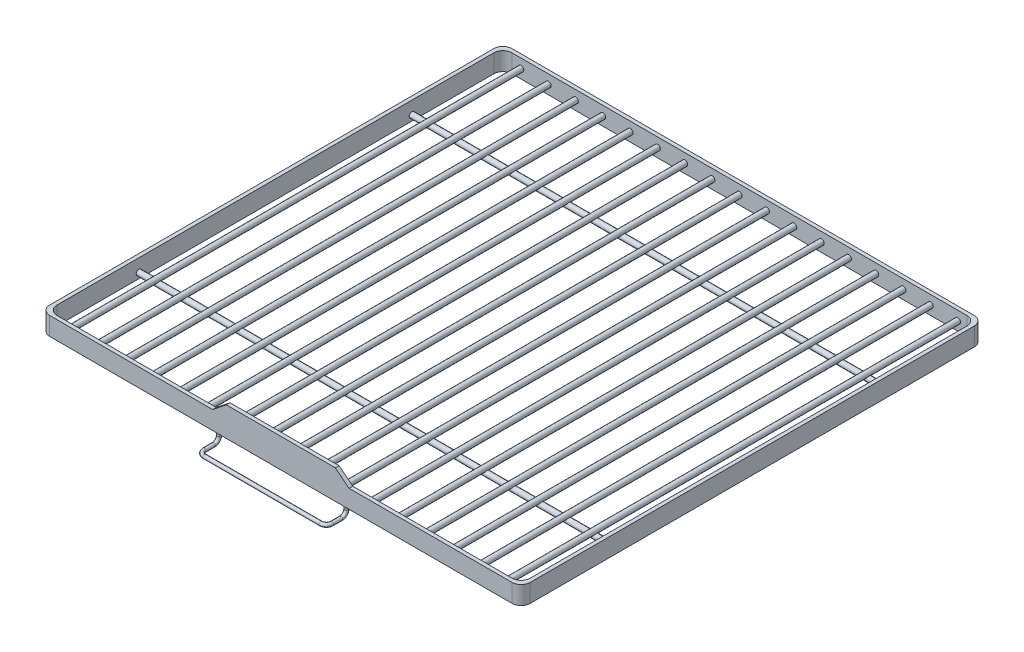
from build123d import *
from build123d.topology import SkipClean

# Parameters (mm, degrees)
SKETCH1_W           = 528
SKETCH1_H           = 508
SKETCH1_W_2         = 520
SKETCH1_H_2         = 500
BOSS_EXTRUDE1_DEPTH = 20
BOSS_EXTRUDE2_DEPTH = 4
FILLET1_R           = 10
SKETCH3_R           = 3
BOSS_EXTRUDE3_DEPTH = 520
BOSS_EXTRUDE4_REACH = 571.856
SKETCH4_R           = 3
LPATTERN1_COUNT     = 9
LPATTERN1_PITCH     = 30
LPATTERN2_COUNT     = 9
LPATTERN2_PITCH     = 30
SWEEP1_PROFILE_R    = 2
SWEEP2_PROFILE_R    = 2


with BuildPart() as part:
    # Sketch1 → Boss-Extrude1 (new body)
    with BuildSketch(Plane(origin=(0, 0, 0), x_dir=(1, 0, 0), z_dir=(0, 1, 0))):
        Rectangle(SKETCH1_W, SKETCH1_H)
        Rectangle(SKETCH1_W_2, SKETCH1_H_2, mode=Mode.SUBTRACT)
    extrude(amount=BOSS_EXTRUDE1_DEPTH)

    # Sketch2 → Boss-Extrude2 (add)
    with BuildSketch(Plane.XY.offset(254)):
        Polygon((60, 32), (-60, 32), (-75, 20), (75, 20), align=None)
    extrude(amount=-BOSS_EXTRUDE2_DEPTH)

    # Fillet1
    fillet1_edges = [part.edges().sort_by_distance(p)[0] for p in [
        (260, 10, 250),
        (260, 10, -250),
        (-260, 10, -250),
        (-260, 10, 250),
        (264, 10, -254),
        (264, 10, 254),
        (-264, 10, 254),
        (-264, 10, -254),
    ]]
    fillet(fillet1_edges, radius=FILLET1_R)

    # Sketch3 → Boss-Extrude3 (add)
    with BuildSketch(Plane(origin=(-260, 0, 0), x_dir=(0, 0, -1), z_dir=(1, 0, 0))):
        with Locations(Location((-150, 6, 0), (0, 0, 180))):
            Circle(SKETCH3_R)
        with Locations(Location((150, 6, 0), (0, 0, 180))):
            Circle(SKETCH3_R)
    extrude(amount=BOSS_EXTRUDE3_DEPTH)

    # Boss-Extrude4: up to this face of the body (flat: up to its plane)
    boss_extrude4_end = Plane(part.part.faces().sort_by_distance((0, 12.199655766, 250))[0])
    # Sketch4 → Boss-Extrude4 (add, up to the picked face)
    with BuildSketch(Plane.XY.offset(-250), mode=Mode.PRIVATE) as boss_extrude4_sk1:
        with Locations(Location((0, 10, 0), (0, 0, 180))):
            Circle(SKETCH4_R)
    boss_extrude4_tool1 = split(extrude(boss_extrude4_sk1.sketch, amount=BOSS_EXTRUDE4_REACH, mode=Mode.PRIVATE), bisect_by=boss_extrude4_end, keep=Keep.BOTH, mode=Mode.PRIVATE)
    boss_extrude4 = boss_extrude4_tool1.solids().sort_by(Axis((0, 10, -250), (0, 0, 1)))[0]
    add(boss_extrude4)

    # LPattern1: Boss-Extrude4 ×9
    with Locations(*[(i * LPATTERN1_PITCH, 0, 0) for i in range(1, LPATTERN1_COUNT)]):
        add(boss_extrude4)

    # LPattern2: Boss-Extrude4 ×9
    with Locations(*[(-i * LPATTERN2_PITCH, 0, 0) for i in range(1, LPATTERN2_COUNT)]):
        add(boss_extrude4)

    # Sweep1: sweep along a path in Sketch5
    with BuildLine(Plane(origin=(70, 0, 0), x_dir=(0, 0, -1), z_dir=(1, 0, 0))) as sweep1_path:
        Line((-252, 0), (-252, -3))
        ThreePointArc((-252, -3), (-253.757359313, -7.242640687), (-258, -9))
        Line((-258, -9), (-264, -9))
    # Sweep1 profile (on start of the path) → Sweep1 (sweep)
    with BuildSketch(Plane(origin=(70, 0, 252), x_dir=(0, 0, -1), z_dir=(0, -1, 0))):
        Circle(SWEEP1_PROFILE_R)
    sweep1 = sweep(path=sweep1_path.line)

    # Mirror1: Sweep1 across plane
    add(sweep1.mirror(Plane(origin=(0, 0, 0), x_dir=(0, 0, 1), z_dir=(1, 0, 0))))

    # Sweep2: sweep along a path in Sketch43
    with SkipClean():  # the faces are left unmerged after this step: merging them gives an invalid solid
        with BuildLine(Plane(origin=(0, -9, 0), x_dir=(1, 0, 0), z_dir=(0, 1, 0))) as sweep2_path:
            Line((-70, -264), (-70, -268))
            ThreePointArc((-70, -268), (-68.242640687, -272.242640687), (-64, -274))
            Line((-64, -274), (64, -274))
            ThreePointArc((64, -274), (68.242640687, -272.242640687), (70, -268))
            Line((70, -268), (70, -264))
        # Sweep2 profile (on start of the path) → Sweep2 (sweep)
        with BuildSketch(Plane(origin=(-70, -9, 264), x_dir=(1, 0, 0), z_dir=(0, 0, 1))):
            Circle(SWEEP2_PROFILE_R)
        sweep(path=sweep2_path.line)


solid = part.part
